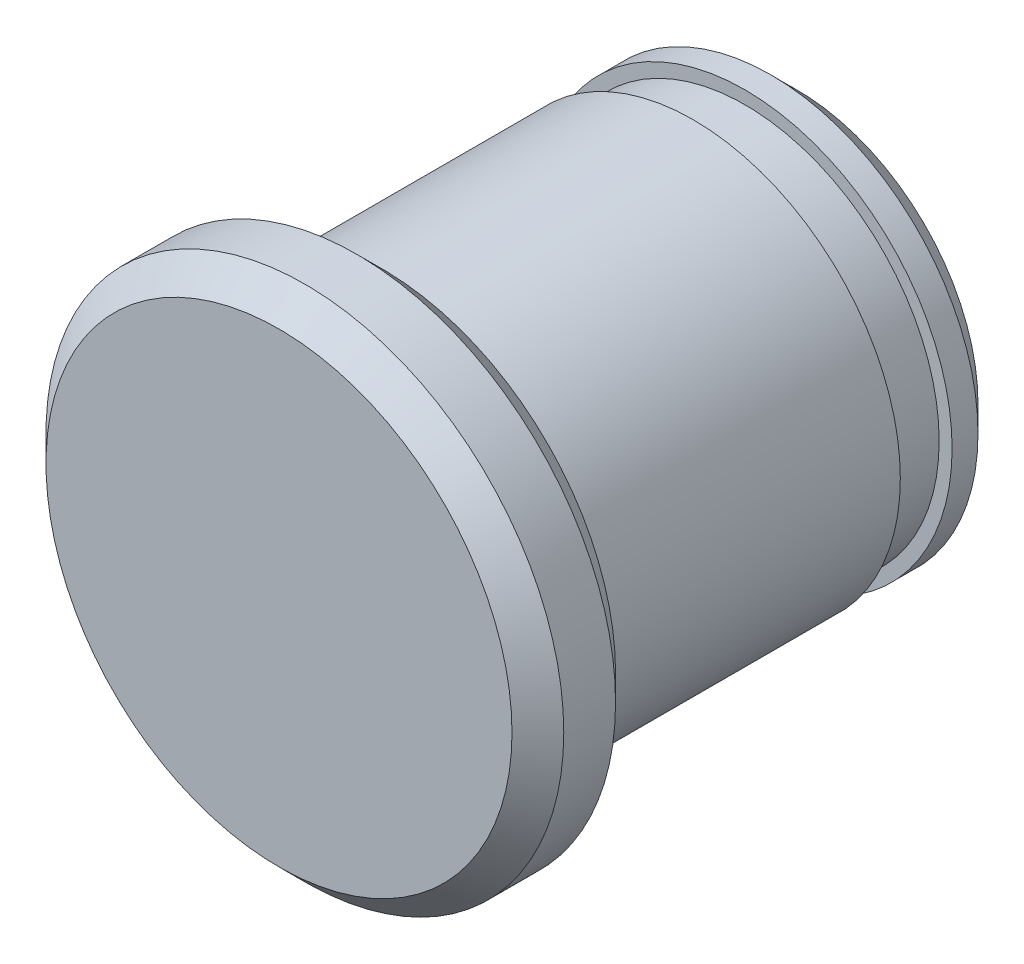
from build123d import *

# Parameters (mm, degrees)
SKETCH1_R           = 4
BOSS_EXTRUDE1_DEPTH = 1
SKETCH2_R           = 3.75
BOSS_EXTRUDE2_DEPTH = 1
SKETCH3_R           = 4
BOSS_EXTRUDE3_DEPTH = 6
SKETCH4_R           = 5
BOSS_EXTRUDE4_DEPTH = 2
CHAMFER1_SIZE       = 0.5


with BuildPart() as part:
    # Sketch1 → Boss-Extrude1 (new body)
    with BuildSketch(Plane.XY):
        Circle(SKETCH1_R)
    extrude(amount=BOSS_EXTRUDE1_DEPTH)

    # Sketch2 → Boss-Extrude2 (add)
    with BuildSketch(Plane.XY.offset(1)):
        Circle(SKETCH2_R)
    extrude(amount=BOSS_EXTRUDE2_DEPTH)

    # Sketch3 → Boss-Extrude3 (add)
    with BuildSketch(Plane.XY.offset(2)):
        Circle(SKETCH3_R)
    extrude(amount=BOSS_EXTRUDE3_DEPTH)

    # Sketch4 → Boss-Extrude4 (add)
    with BuildSketch(Plane.XY.offset(8)):
        Circle(SKETCH4_R)
    extrude(amount=BOSS_EXTRUDE4_DEPTH)

    # Chamfer1
    chamfer1_edges = [part.edges().sort_by_distance(p)[0] for p in [
        (-5, 0, 8),
        (-5, 0, 10),
        (-4, 0, 0),
    ]]
    chamfer(chamfer1_edges, length=CHAMFER1_SIZE)


solid = part.part
